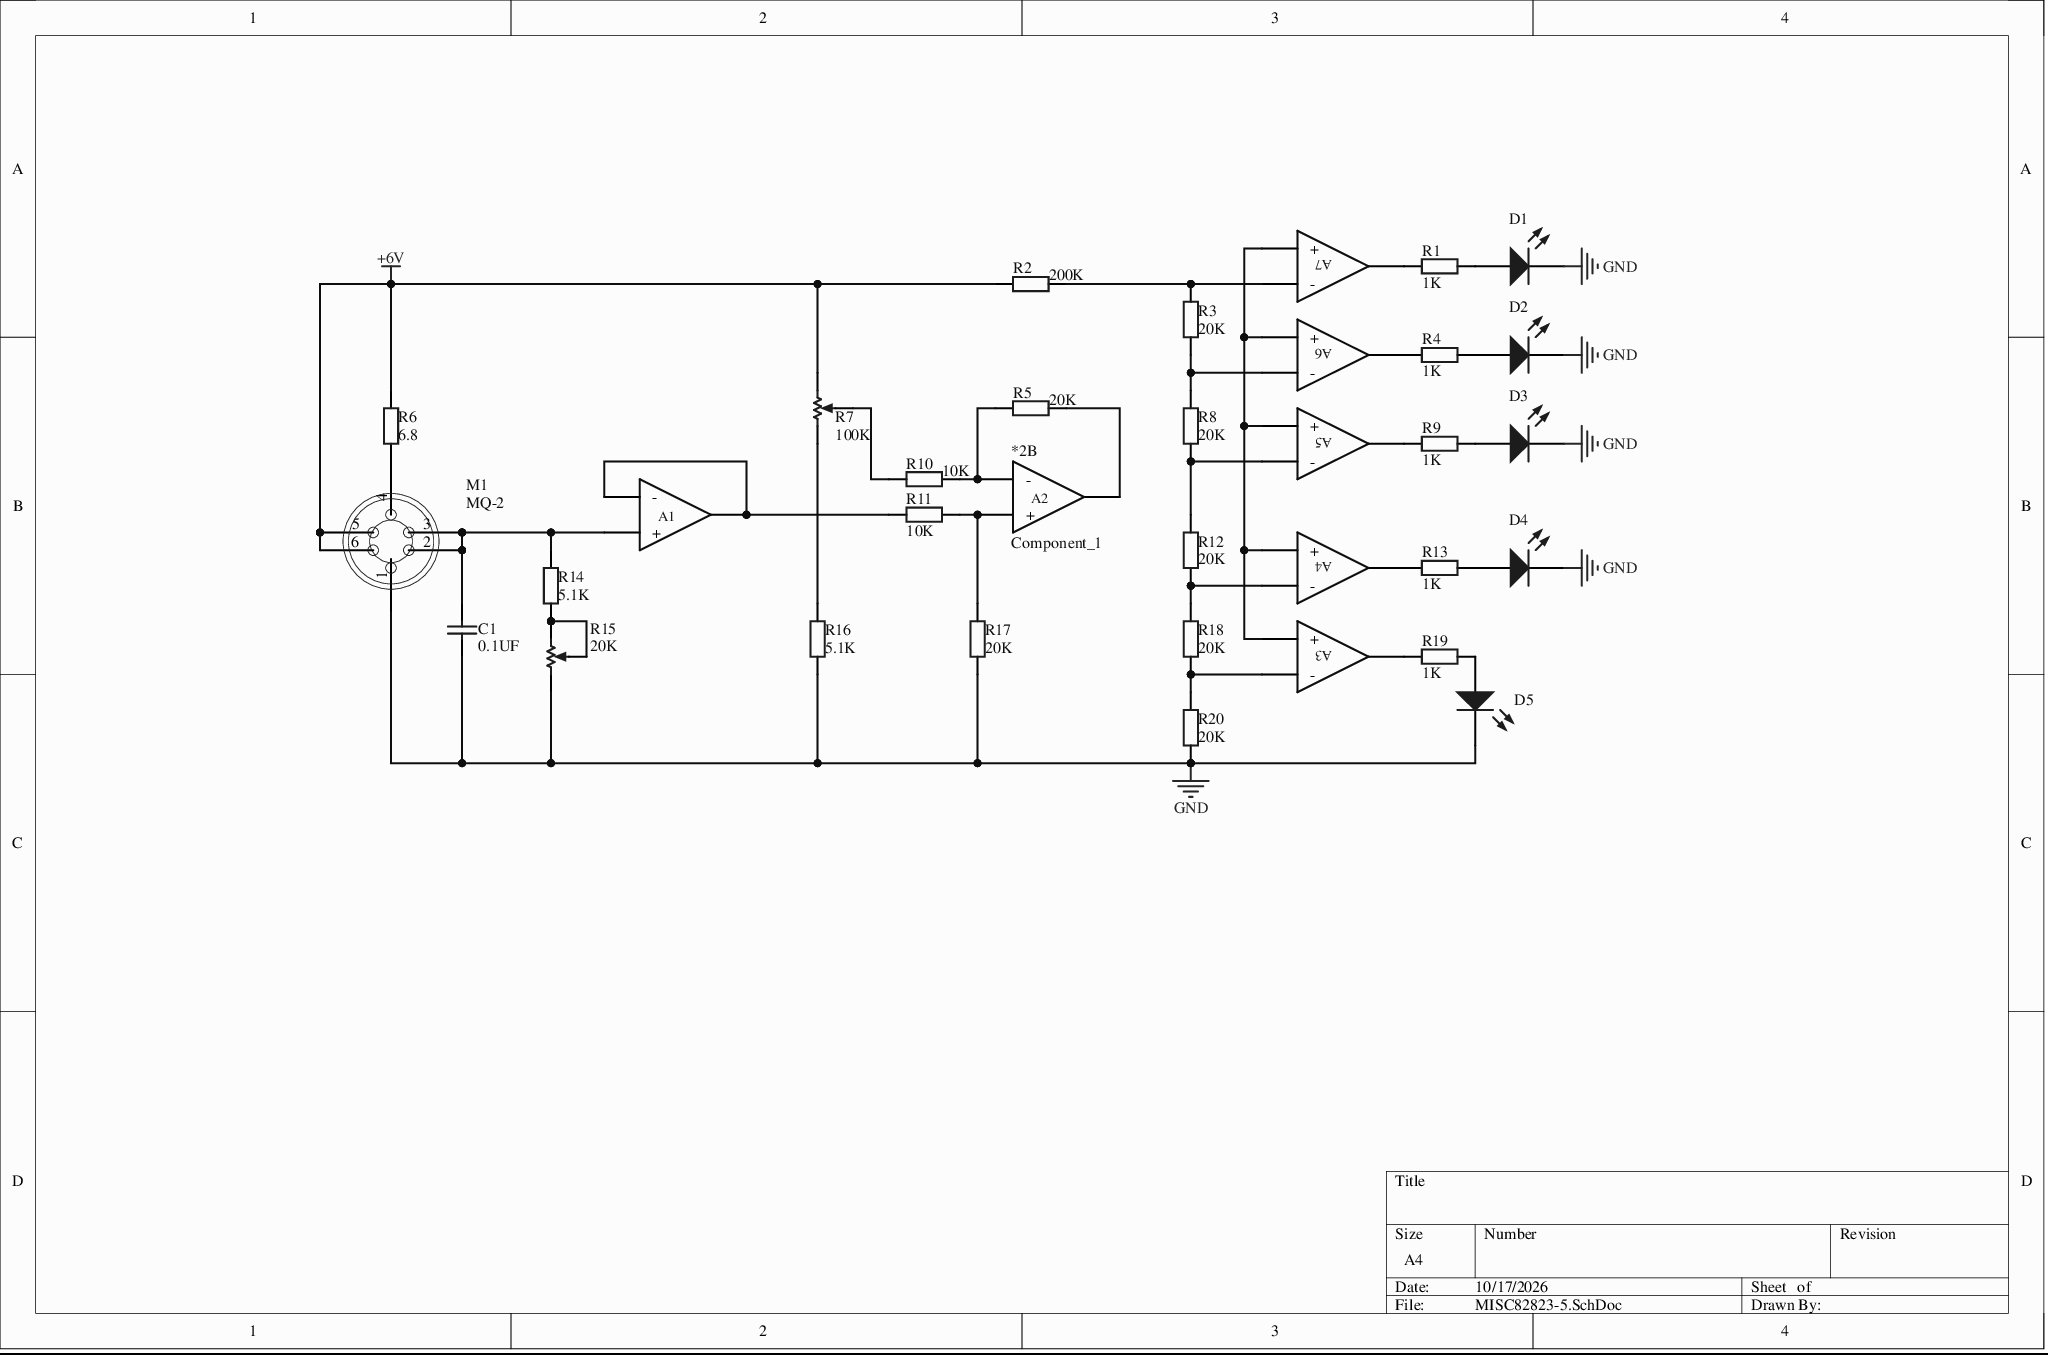
[diagram p0: MISC82823-5.SchDoc]
# Altium project MISC82823-8.PrjPcb
1 sheet, 29 parts. Net scope: global (net labels, ports and power ports of the same name join across sheets).
Board file: MISC82823.PcbDoc

## Sheet MISC82823-5.SchDoc
size A4

### Parts
*1  Component_2  [DIP14]  (value not drawn)  (parts A,B,C,D of 4)
*2  Component_1  [DIP14]  (value not drawn)  (parts A,B,C of 3)
C1  0.1UF  [RAD-0.1]
D1  LED3  [LED3MM]  (value not drawn)
D2  LED3  [LED3MM]  (value not drawn)
D3  LED3  [LED3MM]  (value not drawn)
D4  LED3  [LED3MM]  (value not drawn)
D5  LED3  [LED3MM]  (value not drawn)
M1  MQ-2  [MQ-2]
R1  1K  [AXIAL-0.4]
R2  200K  [AXIAL-0.4]
R3  20K  [AXIAL-0.4]
R4  1K  [AXIAL-0.4]
R5  20K  [AXIAL-0.4]
R6  6.8  [AXIAL-0.4]
R7  100K  [VR5]
R8  20K  [AXIAL-0.4]
R9  1K  [AXIAL-0.4]
R10  10K  [AXIAL-0.4]
R11  10K  [AXIAL-0.4]
R12  20K  [AXIAL-0.4]
R13  1K  [AXIAL-0.4]
R14  5.1K  [AXIAL-0.4]
R15  20K  [VR5]
R16  5.1K  [AXIAL-0.4]
R17  20K  [AXIAL-0.4]
R18  20K  [AXIAL-0.4]
R19  1K  [AXIAL-0.4]
R20  20K  [AXIAL-0.4]

### Nets
+6V: M1.5(A2) M1.6(B2) R2.2 R6.2 R7.2(BOT)
GND: C1.1 D1.2(K) D2.2(K) D3.2(K) D4.2(K) D5.2(K) M1.1(H1) R15.1(TOP) R16.1 R17.1 R20.2
Net*1_2: *1.2(-) R12.2 R18.1
Net*1_3: *1.3(+) *1.6(+) *1.9(+) *1.12(+) *2.9(+)
Net*1_4: *1.4(+) R13.1
Net*1_5: *1.5(-) R8.2 R12.1
Net*1_7: *1.7 R9.1
Net*1_8: *1.8(-) R3.2 R8.1
Net*1_10: *1.10(+) R4.1
Net*1_11: *1.11(-) R2.1 R3.1
Net*1_13: *1.13(+) R1.1
Net*2_2: *2.2(-) *2.4(+) R11.2
Net*2_3: *2.3(+) C1.2 M1.2 M1.3(A1) R14.2
Net*2_5: *2.5(-) R5.2 R10.1
Net*2_6: *2.6(+) R11.1 R17.2
Net*2_7: *2.7(+) R5.1
Net*2_8: *2.8(-) R18.2 R20.1
Net*2_10: *2.10(+) R19.1
NetD1_1: D1.1(A) R1.2
NetD2_1: D2.1(A) R4.2
NetD3_1: D3.1(A) R9.2
NetD4_1: D4.1(A) R13.2
NetD5_1: D5.1(A) R19.2
NetM1_4: M1.4(H2) R6.1
NetR7_1: R7.1(TOP) R16.2
NetR7_3: R7.3(TAP) R10.2
NetR14_1: R14.1 R15.2(BOT) R15.3(TAP)

### Library data of the parts
C1 = Cap: Capacitor; Value: 100pF; Published: 8-Jun-2000; LatestRevisionDate: 17-Jul-2002; LatestRevisionNote: Re-released for DXP Platform.; PackageReference: RAD-0.3; PackageDescription: Radial Cap, Thru-Hole; 2 Leads; 0.3 in Pin Spacing; Publisher: Altium Limited
D1-D5 = LED3: Typical BLUE SiC LED; Published: 8-Jun-2000; LatestRevisionDate: 17-Dec-2003; LatestRevisionNote: PCB Footprint replaced.; DatasheetVersion: 16-Apr-2002; PackageVersion: 16-Apr-2002; PackageReference: 3.5X2.8X1.9; PackageDescription: SM LED; 2 C-Bend Leads; Body 3.5 x 2.8 x 1.9 mm, inc leads (LxWxH typ); Publisher: Altium Limited
M1 = MQ-2: Gas sensor
R1 R4 R9 R13 R19 = Res2: Resistor; Published: 8-Jun-2000; LatestRevisionDate: 17-Jul-2002; LatestRevisionNote: Re-released for DXP Platform.; PackageReference: AXIAL-0.4; PackageDescription: Axial Device, Thru-Hole; 2 Leads; 0.4 in Pin Spacing; Value: 1K; Publisher: Altium Limited
R2 R3 R5 R6 R8 R10-R12 R14 R16-R18 R20 = Res2: Resistor; Value: 1K; Published: 8-Jun-2000; LatestRevisionDate: 17-Jul-2002; LatestRevisionNote: Re-released for DXP Platform.; PackageReference: AXIAL-0.4; PackageDescription: Axial Device, Thru-Hole; 2 Leads; 0.4 in Pin Spacing; Publisher: Altium Limited
R7 R15 = RPot: Potentiometer; Sim Note: Enter the Resistance value and the set point into parameter fields.; Set Position: 0.5; Value: 1K; Published: 8-Jun-2000; LatestRevisionDate: 17-Jul-2002; LatestRevisionNote: Re-released for DXP Platform.; PackageReference: VR5; PackageDescription: Variable Resistor, Thru-Hole; 3 Leads; Publisher: Altium Limited